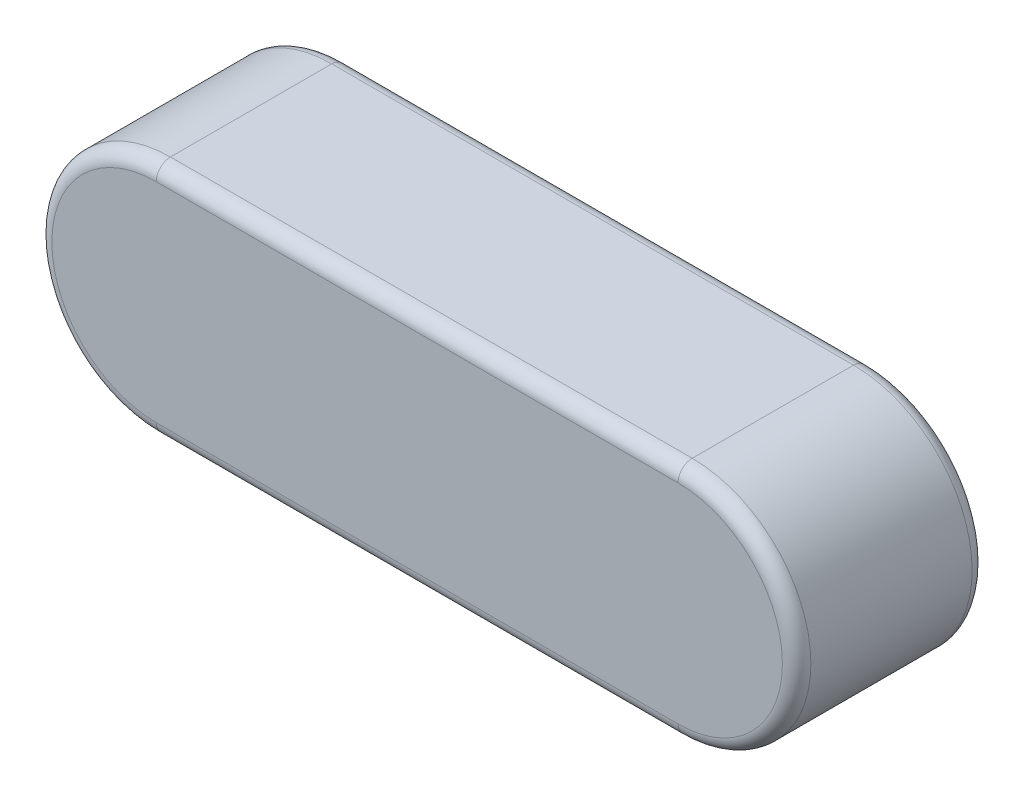
from build123d import *

# Parameters (mm, degrees)
EXTRUDE_523_DEPTH = 8
FILLET_1_R        = 0.6


with BuildPart() as part:
    # 草图1 → Extrude 523 (new body)
    with BuildSketch(Plane.XY):
        with BuildLine():
            Line((-11, 5), (11, 5))
            ThreePointArc((11, 5), (16, 0), (11, -5))
            Line((11, -5), (-11, -5))
            ThreePointArc((-11, -5), (-16, 0), (-11, 5))
        make_face()
    extrude(amount=EXTRUDE_523_DEPTH)

    # 圆角1
    fillet_1_edges = [part.edges().sort_by_distance(p)[0] for p in [
        (16, 0, 8),
        (0, 5, 8),
        (-16, 0, 8),
        (0, 5, 0),
        (16, 0, 0),
        (0, -5, 0),
        (-16, 0, 0),
        (0, -5, 8),
    ]]
    fillet(fillet_1_edges, radius=FILLET_1_R)


solid = part.part
